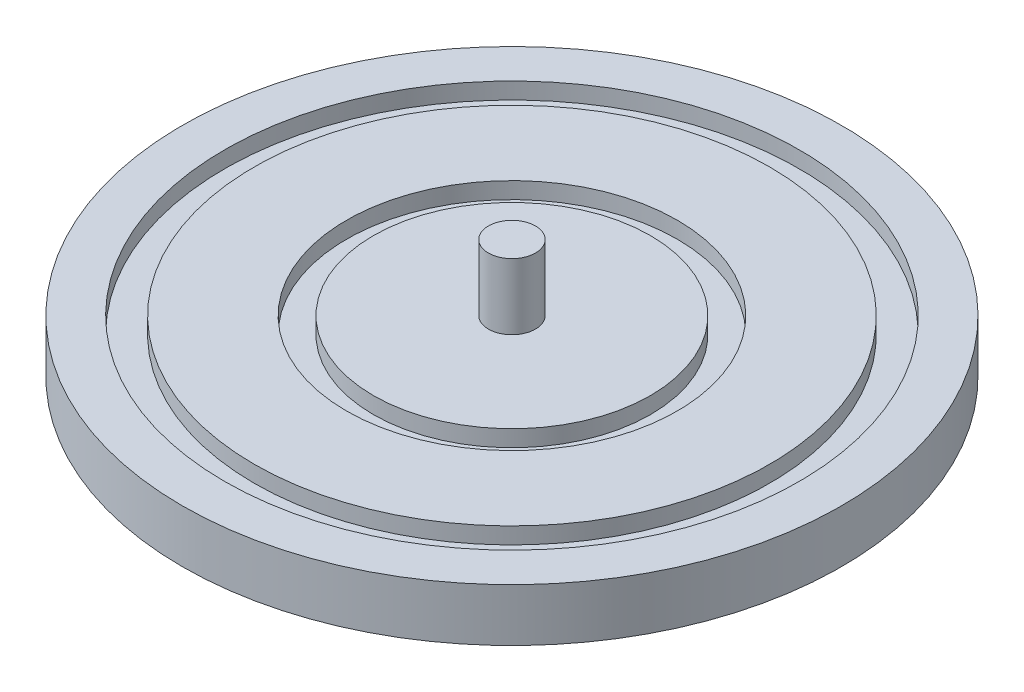
from build123d import *

# Parameters (mm, degrees)
SKETCH_1_R          = 20
EXTRUDE_1_DEPTH     = 3.2
SKETCH_2_R          = 5
EXTRUDE_2_DEPTH     = 6
SKETCH_3_R          = 11.669468733
SKETCH_3_R_2        = 9.545408708
CUT_EXTRUDE_1_DEPTH = 1
SKETCH_4_R          = 1.425
EXTRUDE_3_DEPTH     = 4
SKETCH_5_R          = 17.435273898
SKETCH_5_R_2        = 15.634190673
CUT_EXTRUDE_2_DEPTH = 1
SKETCH_6_R          = 10.034081131
SKETCH_6_R_2        = 8.408881881
CUT_EXTRUDE_3_DEPTH = 1


with BuildPart() as part:
    # 草图1 → 凸台-拉伸1 (new body)
    with BuildSketch(Plane(origin=(0, 0, 0), x_dir=(1, 0, 0), z_dir=(0, 1, 0))):
        with Locations(Location((0, 0, 0), (0, 0, 270))):
            Circle(SKETCH_1_R)
    extrude(amount=EXTRUDE_1_DEPTH)

    # 草图2 → 凸台-拉伸2 (add)
    with BuildSketch(Plane.XZ):
        with Locations(Location((0, 0, 0), (0, 0, 270))):
            Circle(SKETCH_2_R)
    extrude(amount=EXTRUDE_2_DEPTH)

    # 草图3 → 切除-拉伸1 (cut)
    with BuildSketch(Plane.XZ):
        with Locations(Location((0, 0, 0), (0, 0, 270))):
            Circle(SKETCH_3_R)
        with Locations(Location((0, 0, 0), (0, 0, 270))):
            Circle(SKETCH_3_R_2, mode=Mode.SUBTRACT)
    extrude(amount=-CUT_EXTRUDE_1_DEPTH, mode=Mode.SUBTRACT)

    # 草图4 → 凸台-拉伸3 (add)
    with BuildSketch(Plane(origin=(0, 3.2, 0), x_dir=(1, 0, 0), z_dir=(0, 1, 0))):
        with Locations(Location((0, 0, 0), (0, 0, 270))):
            Circle(SKETCH_4_R)
    extrude(amount=EXTRUDE_3_DEPTH)

    # 草图5 → 切除-拉伸2 (cut)
    with BuildSketch(Plane(origin=(0, 3.2, 0), x_dir=(1, 0, 0), z_dir=(0, 1, 0))):
        with Locations(Location((0, 0, 0), (0, 0, 270))):
            Circle(SKETCH_5_R)
        with Locations(Location((0, 0, 0), (0, 0, 270))):
            Circle(SKETCH_5_R_2, mode=Mode.SUBTRACT)
    extrude(amount=-CUT_EXTRUDE_2_DEPTH, mode=Mode.SUBTRACT)

    # 草图6 → 切除-拉伸3 (cut)
    with BuildSketch(Plane(origin=(0, 3.2, 0), x_dir=(1, 0, 0), z_dir=(0, 1, 0))):
        with Locations(Location((0, 0, 0), (0, 0, 270))):
            Circle(SKETCH_6_R)
        with Locations(Location((0, 0, 0), (0, 0, 270))):
            Circle(SKETCH_6_R_2, mode=Mode.SUBTRACT)
    extrude(amount=-CUT_EXTRUDE_3_DEPTH, mode=Mode.SUBTRACT)


solid = part.part
